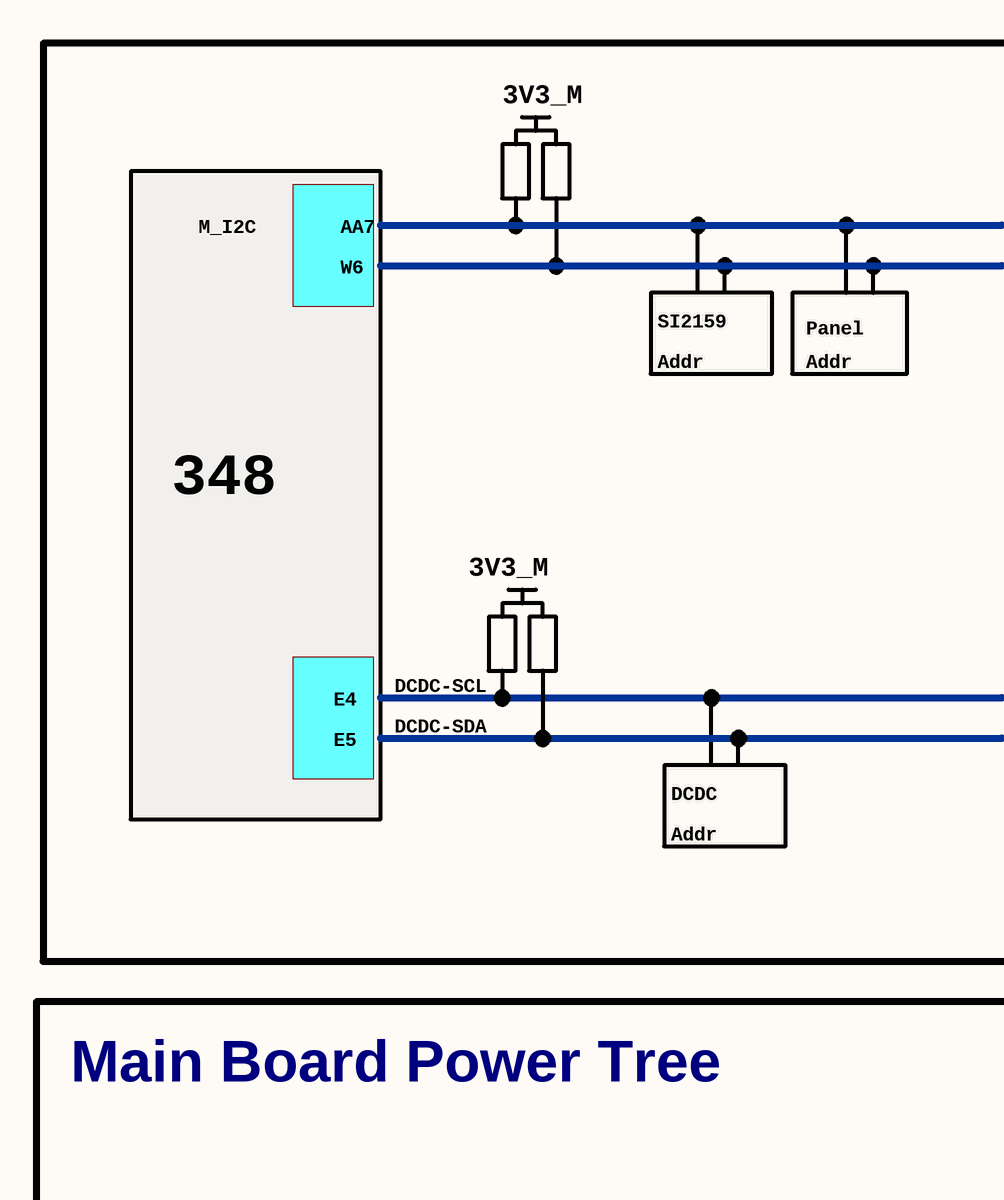
[diagram p0: MISC84395-2.schdoc, top left]
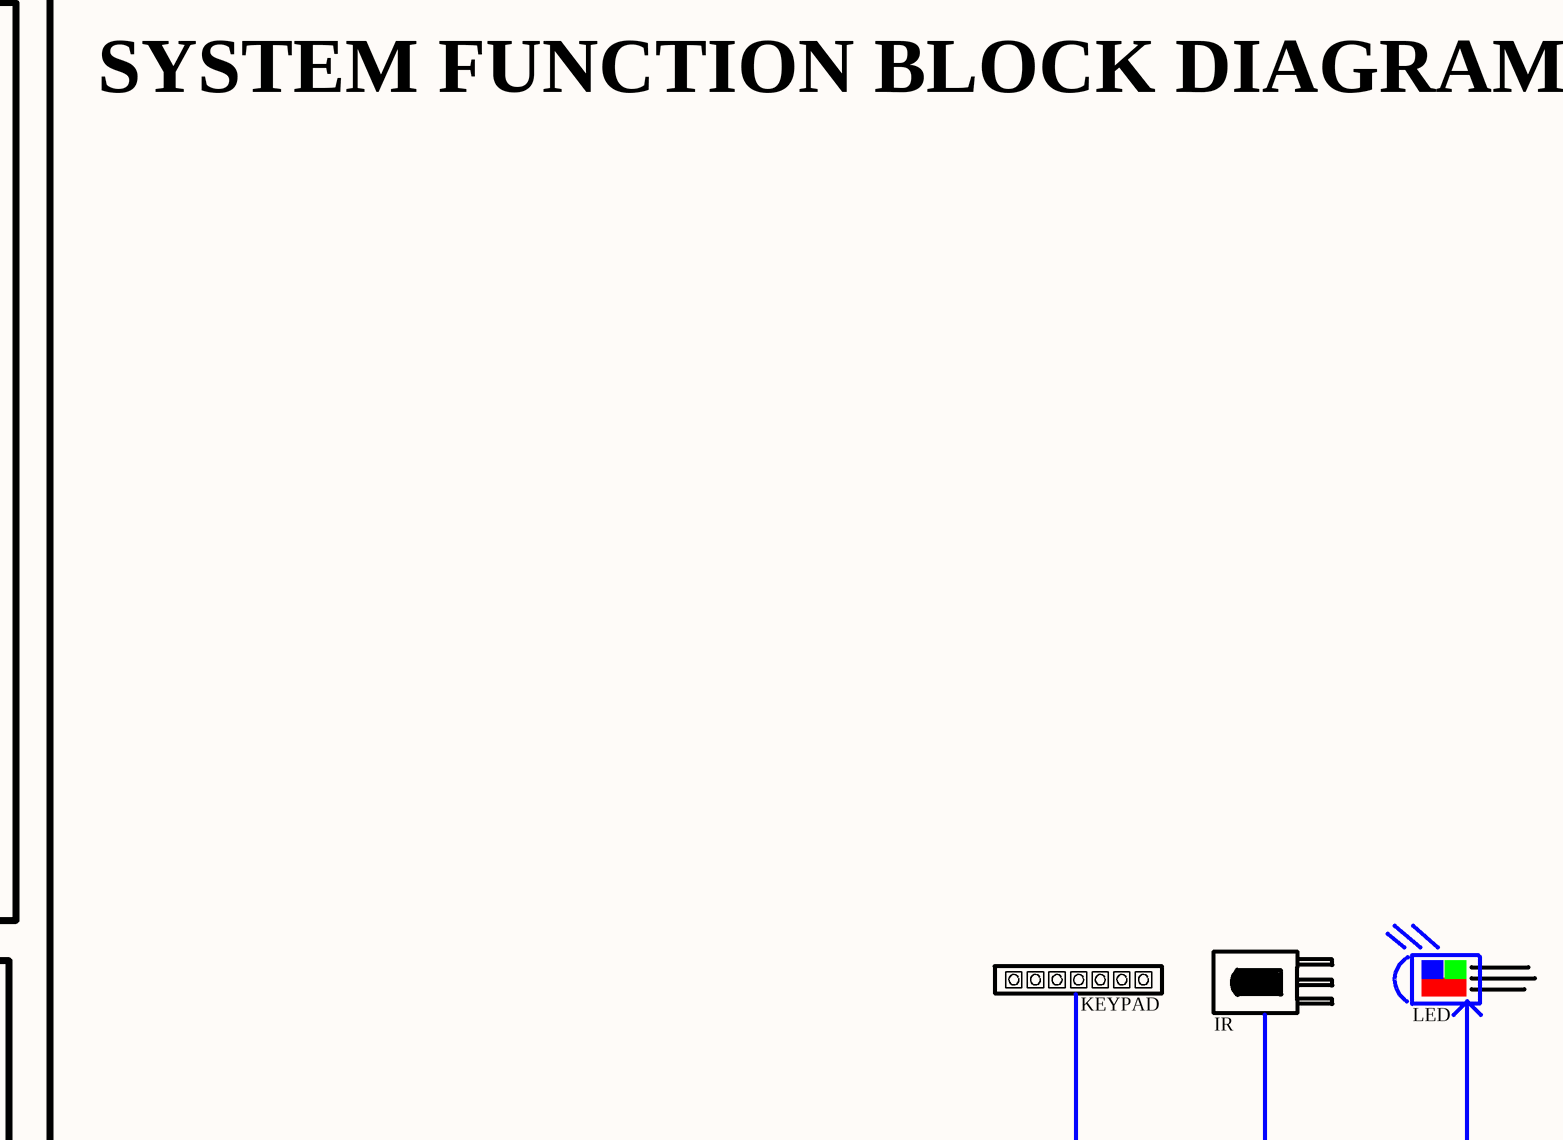
[diagram p1: MISC84395-2.schdoc, top middle]
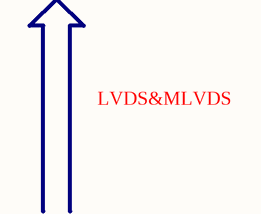
[diagram p2: MISC84395-2.schdoc, top right]
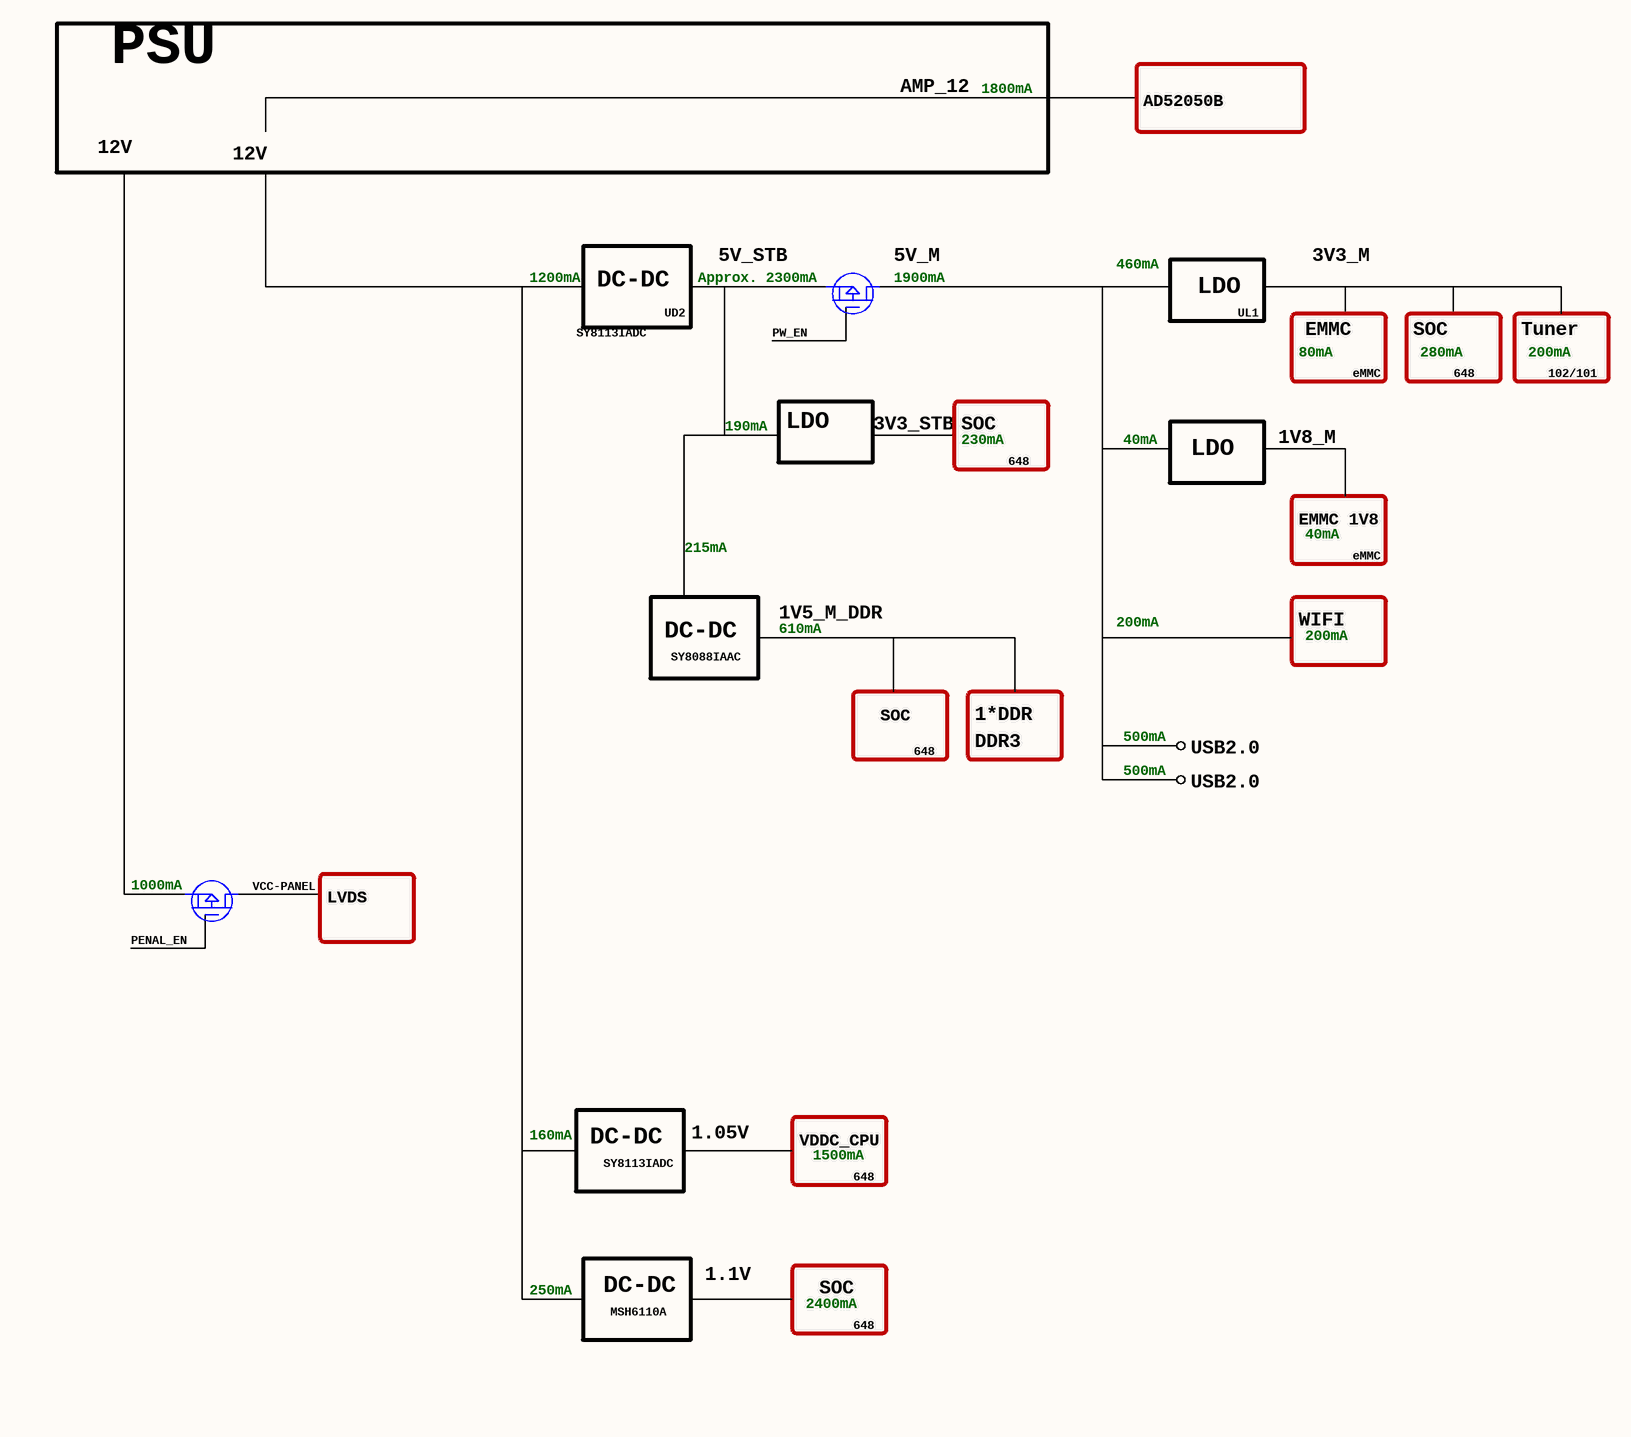
[diagram p3: MISC84395-2.schdoc, bottom left]
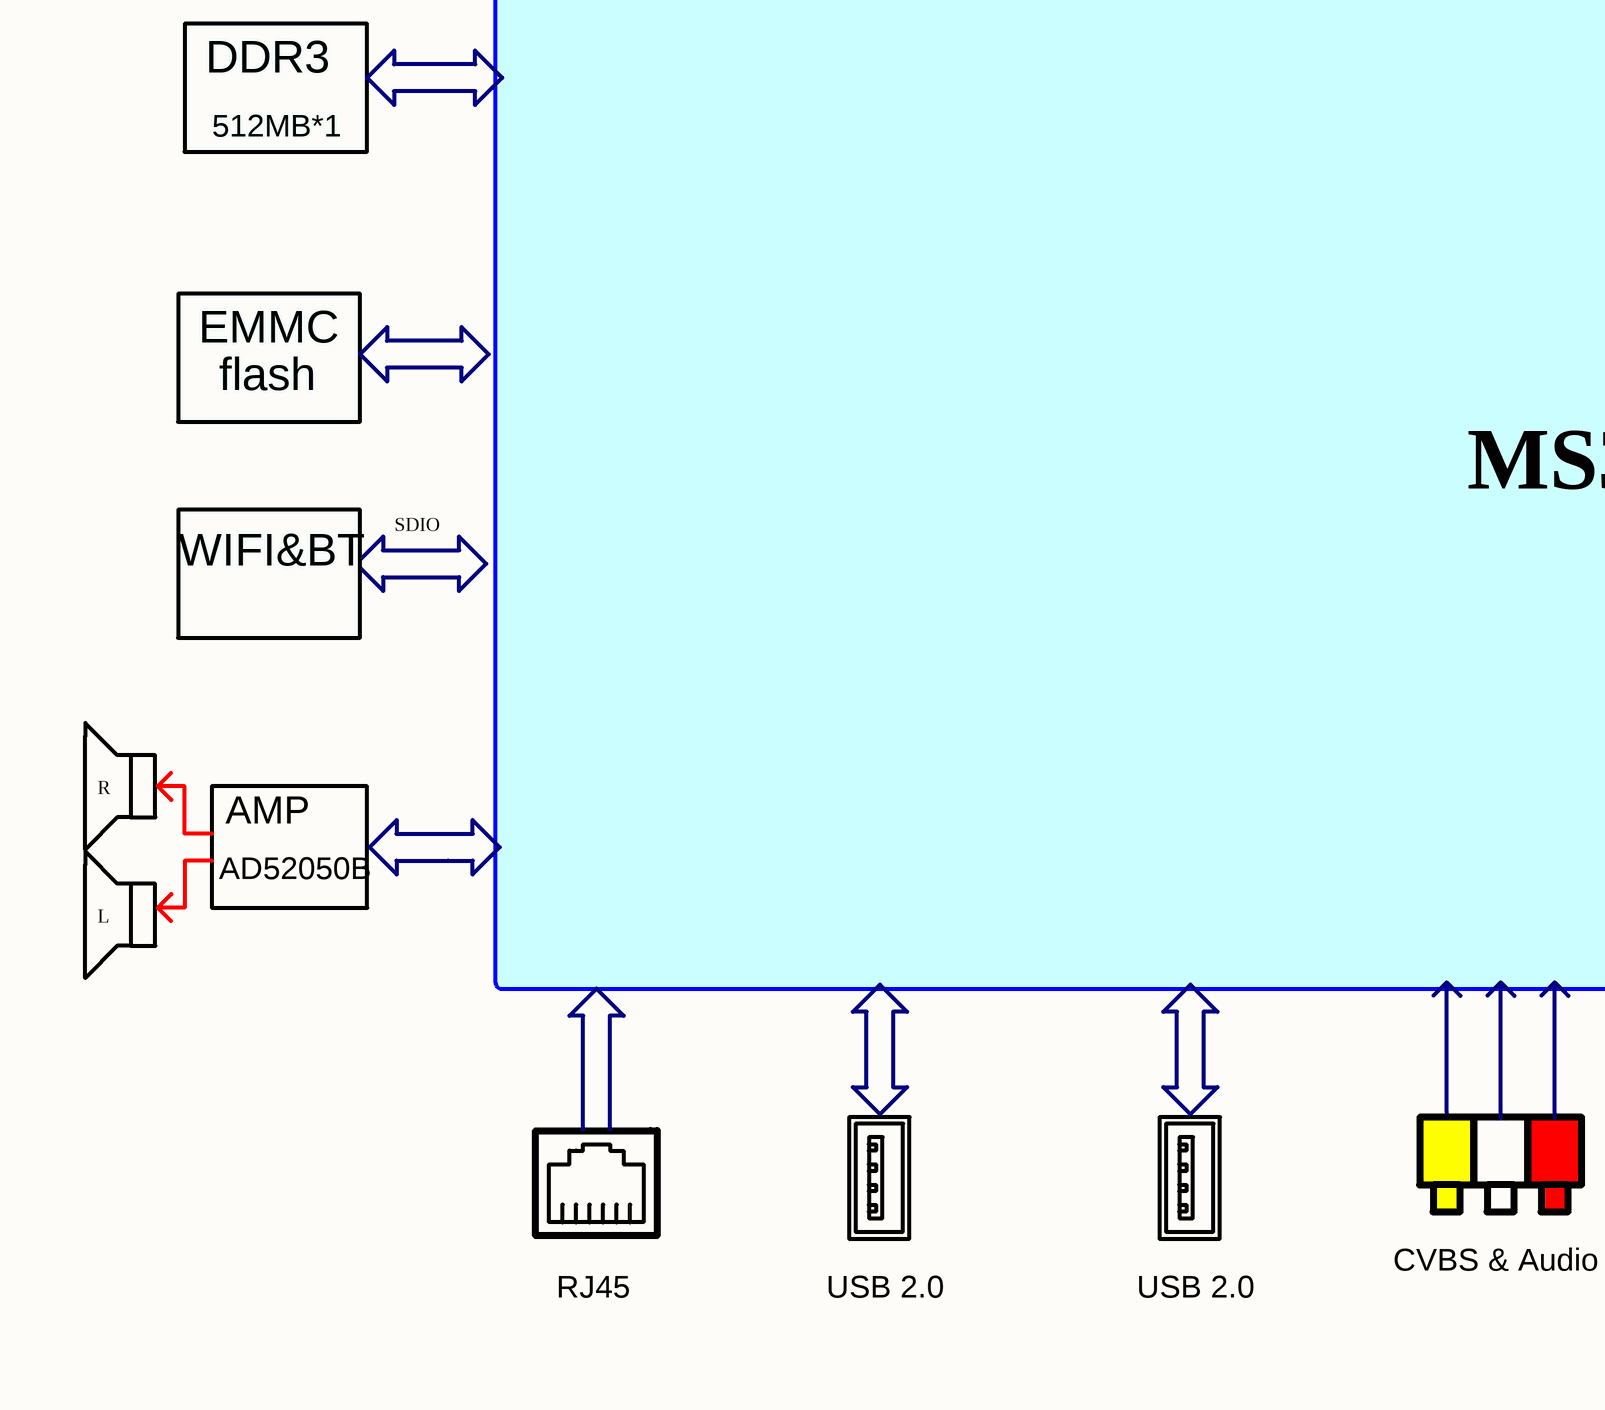
[diagram p4: MISC84395-2.schdoc, bottom middle]
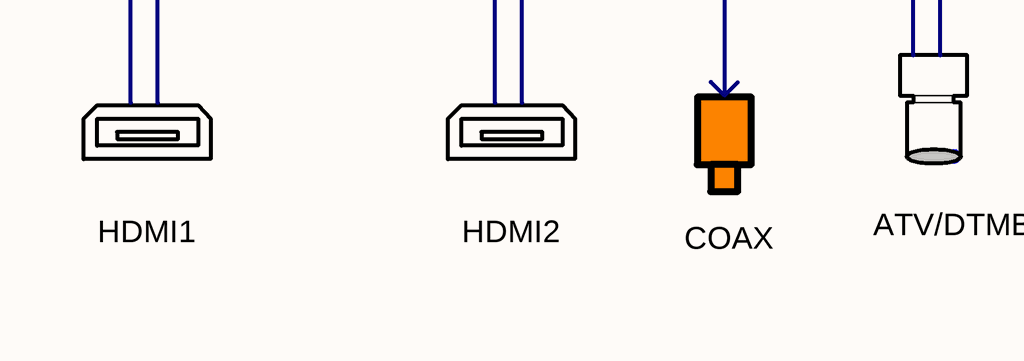
[diagram p5: MISC84395-2.schdoc, bottom right]
# Altium project MISC84395-37.PrjPCB (part 2 of 13)

## Sheet MISC84395-2.schdoc
size 980 x 635 mm